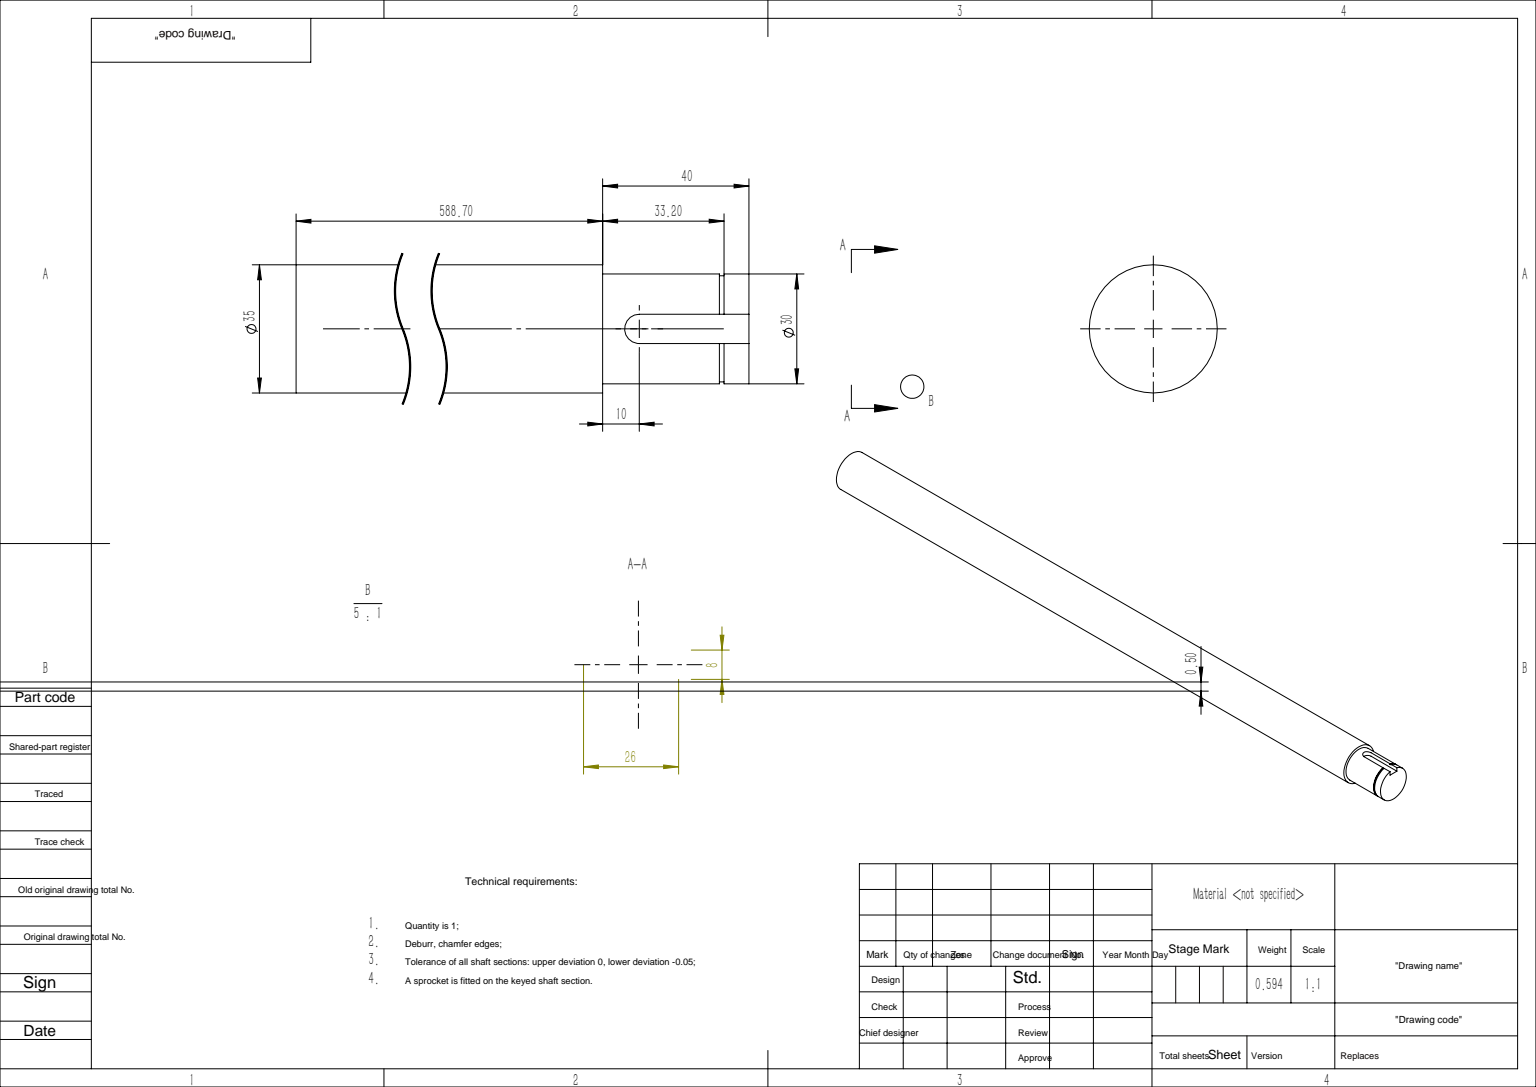
from build123d import *

# Parameters (mm, degrees)
SKETCH_1_R          = 17.5
EXTRUDE_1_DEPTH     = 628.7
CUT_EXTRUDE_START   = -40
SKETCH_3_R          = 17.5
SKETCH_3_R_2        = 15
CUT_EXTRUDE_1_DEPTH = 40
CUT_EXTRUDE_2_DEPTH = 4
CUT_EXTRUDE_START_2 = 31.9
SKETCH_5_R          = 15
SKETCH_5_R_2        = 14.5
CUT_EXTRUDE_3_DEPTH = 1.3


with BuildPart() as part:
    # 草图1 → 凸台-拉伸1 (new body)
    with BuildSketch(Plane(origin=(0, 0, 0), x_dir=(0, 0, -1), z_dir=(1, 0, 0))):
        with Locations(Location((0, 0, 0), (0, 0, 180))):
            Circle(SKETCH_1_R)
    extrude(amount=EXTRUDE_1_DEPTH)

    # 草图3 → 切除-拉伸1 (cut)
    with BuildSketch(Plane(origin=(628.7, 0, 0), x_dir=(0, 0, -1), z_dir=(1, 0, 0)).offset(CUT_EXTRUDE_START)):
        with Locations(Location((0, 0, 0), (0, 0, 180))):
            Circle(SKETCH_3_R)
        Circle(SKETCH_3_R_2, mode=Mode.SUBTRACT)
    extrude(amount=CUT_EXTRUDE_1_DEPTH, mode=Mode.SUBTRACT)

    # 草图4 → 切除-拉伸2 (cut)
    with BuildSketch(Plane(origin=(0, 15, 0), x_dir=(1, 0, 0), z_dir=(0, 1, 0))):
        with BuildLine():
            Line((598.7, 4), (628.7, 4))
            Line((628.7, 4), (628.7, -4))
            Line((628.7, -4), (598.7, -4))
            ThreePointArc((598.7, -4), (594.7, 0), (598.7, 4))
        make_face()
    extrude(amount=-CUT_EXTRUDE_2_DEPTH, mode=Mode.SUBTRACT)

    # 草图5 → 切除-拉伸3 (cut)
    with BuildSketch(Plane(origin=(588.7, 0, 0), x_dir=(0, 0, -1), z_dir=(1, 0, 0)).offset(CUT_EXTRUDE_START_2)):
        Circle(SKETCH_5_R)
        Circle(SKETCH_5_R_2, mode=Mode.SUBTRACT)
    extrude(amount=CUT_EXTRUDE_3_DEPTH, mode=Mode.SUBTRACT)


solid = part.part
